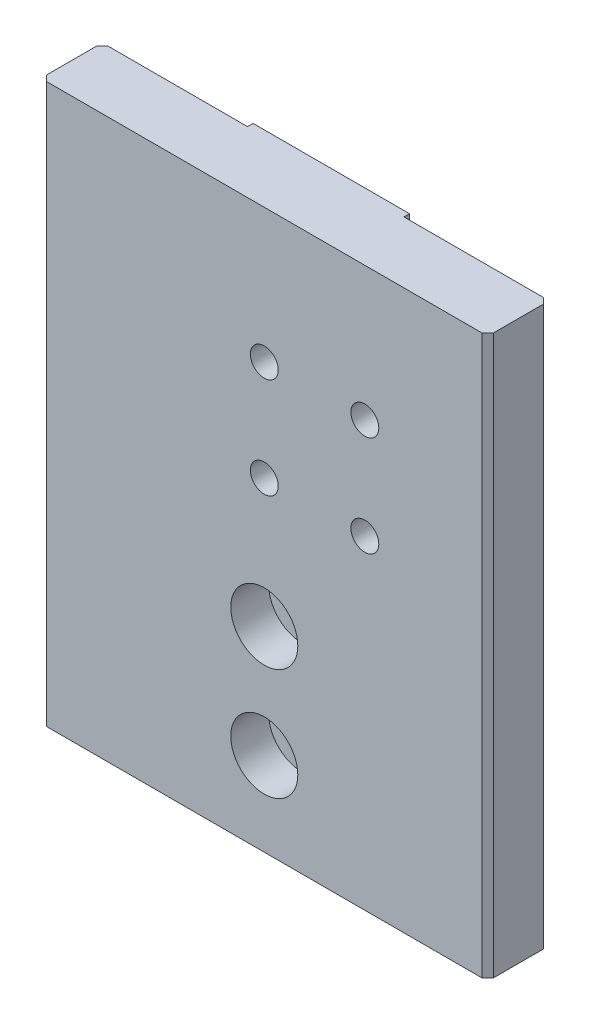
from build123d import *

# Parameters (mm, degrees)
BOSS_EXTRUDE1_DEPTH                                  = 25
CHAMFER1_SIZE                                        = 0.5
HOLE_SIZE_PER_SOCKET_HEAD_CAP_SCREW_TYPE_D           = 3.4
HOLE_SIZE_PER_SOCKET_HEAD_CAP_SCREW_TYPE_CBORE_D     = 6
HOLE_SIZE_PER_SOCKET_HEAD_CAP_SCREW_TYPE_CBORE_DEPTH = 3.4
M3_TAPPED_HOLE1_D                                    = 2.5
M3_TAPPED_HOLE1_DEPTH                                = 7.5
M3_TAPPED_HOLE1_TIP                                  = 0.751075774


with BuildPart() as part:
    # Sketch1 → Boss-Extrude1 (new, symmetric)
    with BuildSketch(Plane(origin=(0, 0, 0), x_dir=(1, 0, 0), z_dir=(0, 1, 0))):
        Polygon((0, 0), (40, 0), (40, 5.5), (27, 5.5), (27, 6), (13, 6), (13, 5.5), (0, 5.5), align=None)
    extrude(amount=BOSS_EXTRUDE1_DEPTH, both=True)

    # Chamfer1
    chamfer1_edges = [part.edges().sort_by_distance(p)[0] for p in [
        (0, 0, -5.5),
        (40, 0, -5.5),
        (40, 0, 0),
        (0, 0, 0),
    ]]
    chamfer(chamfer1_edges, length=CHAMFER1_SIZE)

    # Hole Size per Socket Head Cap Screw Type1 (through all)
    with Locations(Plane.XY):
        with Locations((20, -7.5), (20, -17.5)):
            CounterBoreHole(HOLE_SIZE_PER_SOCKET_HEAD_CAP_SCREW_TYPE_D / 2, HOLE_SIZE_PER_SOCKET_HEAD_CAP_SCREW_TYPE_CBORE_D / 2, HOLE_SIZE_PER_SOCKET_HEAD_CAP_SCREW_TYPE_CBORE_DEPTH)

    # M3 Tapped Hole1
    with Locations(Plane.XY):
        with Locations((20, 13), (29, 13), (20, 4), (29, 4)):
            Hole(M3_TAPPED_HOLE1_D / 2, depth=M3_TAPPED_HOLE1_DEPTH)
            with Locations((0, 0, -(M3_TAPPED_HOLE1_DEPTH + M3_TAPPED_HOLE1_TIP / 2))):  # 118° drill point
                Cone(0, M3_TAPPED_HOLE1_D / 2, M3_TAPPED_HOLE1_TIP, mode=Mode.SUBTRACT)


solid = part.part
